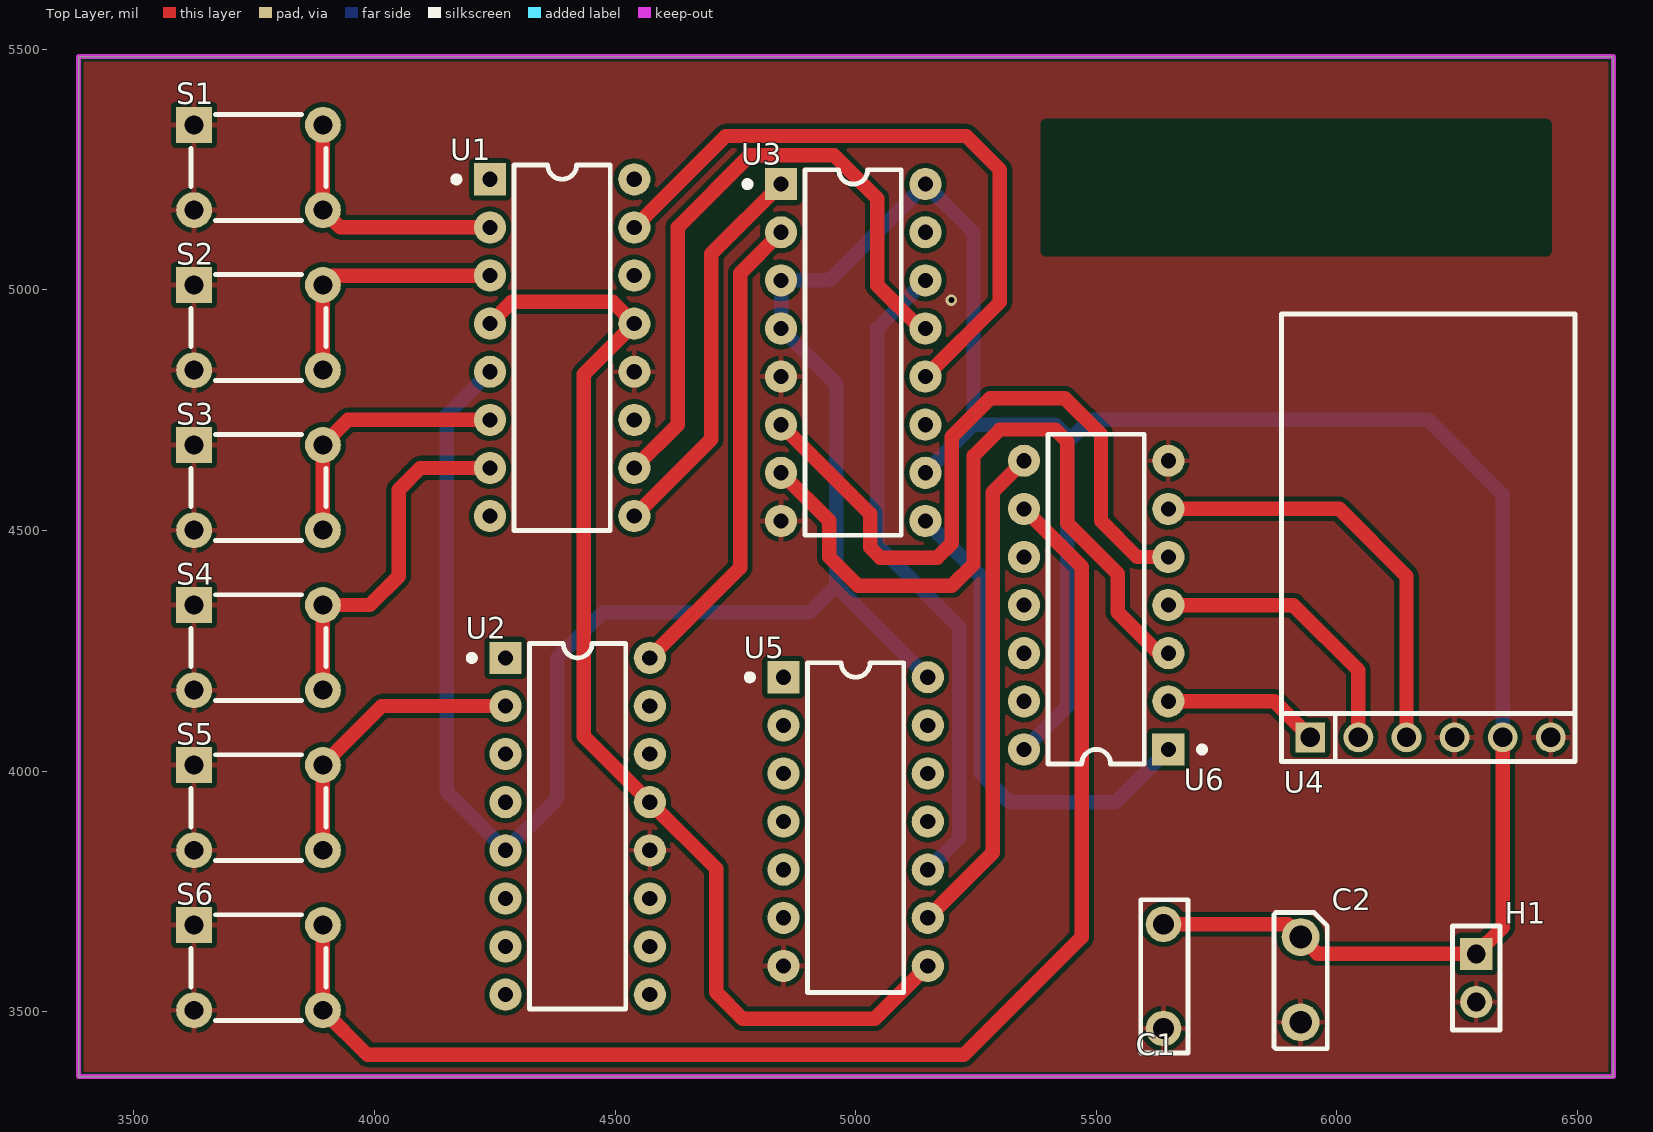
[diagram p0: Top Layer view]
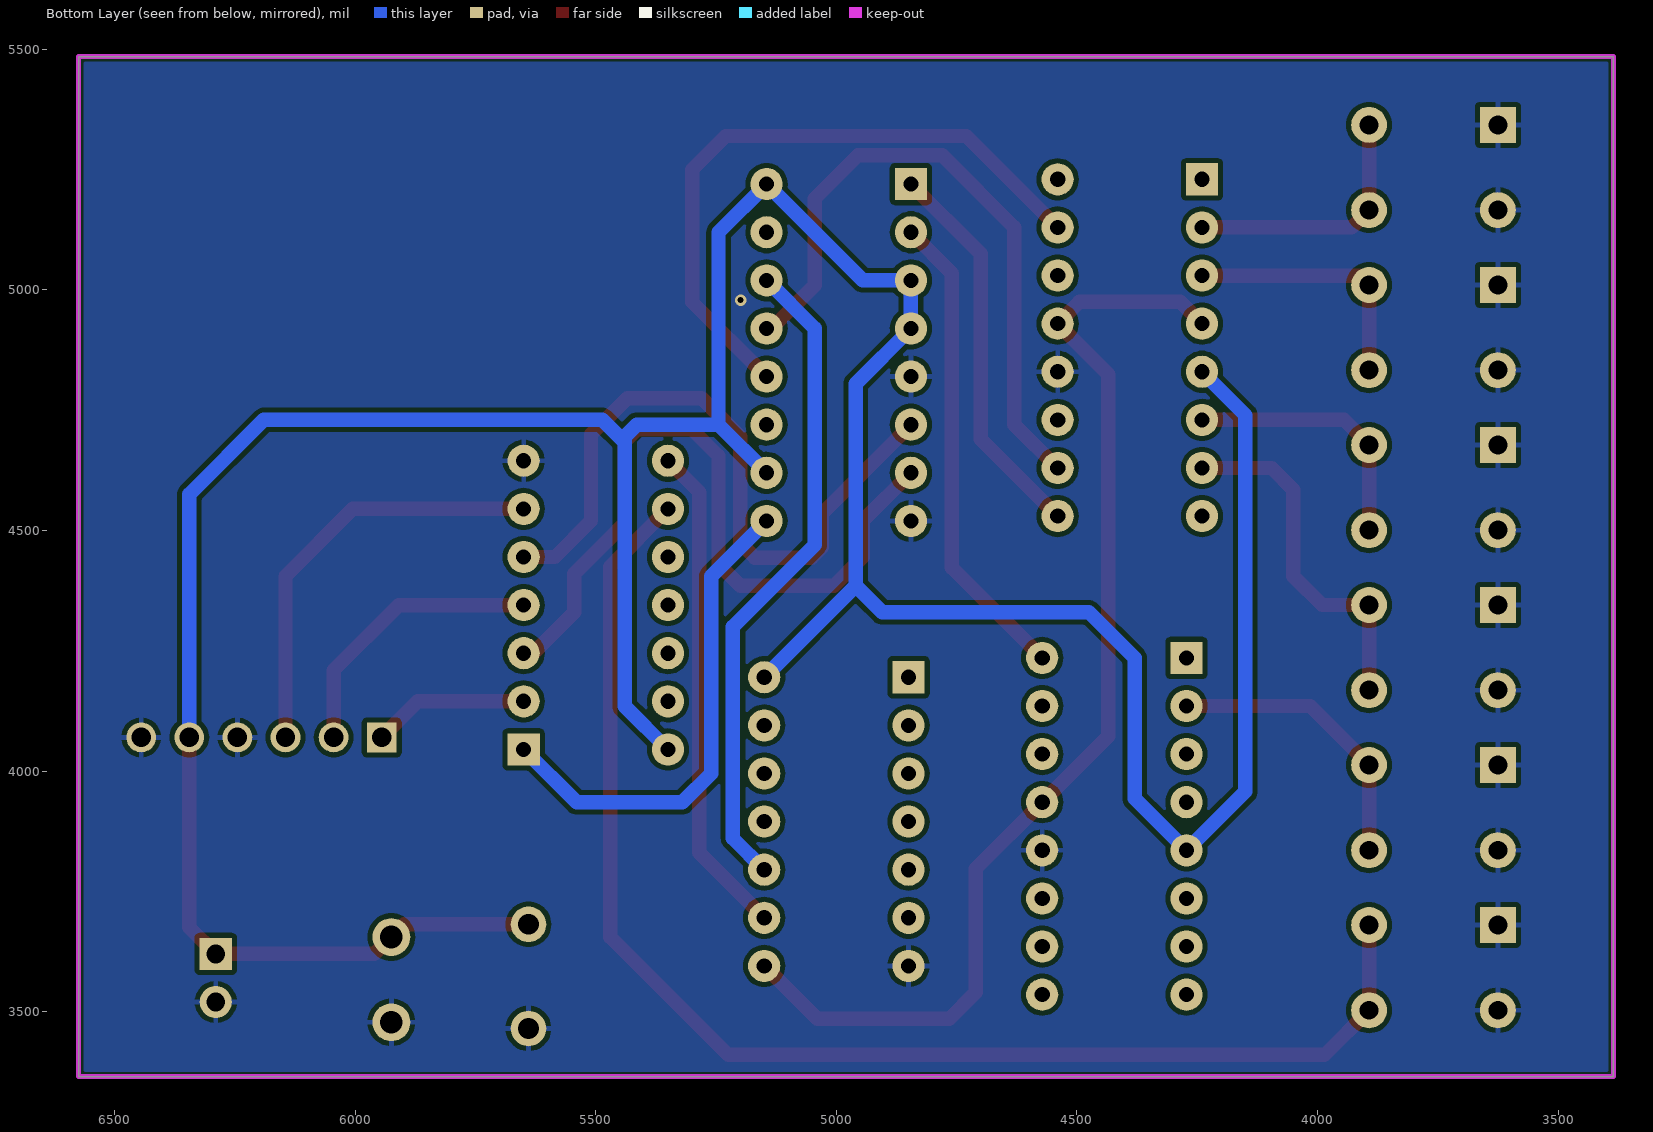
[diagram p1: Bottom Layer view, seen from below]
# Altium PCB MISC51507.pcbdoc
Units mil, origin at the board's own origin, x right, y up, seen from the top; angles counter-clockwise.
Board outline 3190 x 2120 mil, 2 copper layers (Top Layer, Bottom Layer), stack 62.206 mil thick; 15 components, 22 nets, 112 pads, 1 vias.

## Layer stack, top to bottom
Top Solder Mask Layer: solder mask 0.394, Dk 3.3
Top Layer: signal copper 1.379
Dielectric1: surface 59.449, FR4, Dk 4.5
Bottom Layer: signal copper 1.378
Bottom Solder Mask Layer: solder mask 0.394, Dk 3.3

## Board outline
3385,5485 3385,3365 6575,3365 6575,5485

## Design rules (kind name [scope] priority, off if disabled: settings)
BoardOutlineClearance copperThickness2oz_1 [All] p2 off: genericclearance=7.99 ignorepadtopadclearanceinfootprint=FALSE except(0: Arc-SplitContinuation Track-SplitContinuation SMDPad-SplitContinuation THPad-SplitContinuation Via-SplitContinuation Fill-SplitContinuation Region-SplitContinuation Poly-SplitContinuation Text-SplitContinuation Hole-SplitContinuation; 5.98: Arc-CutoutEdge SMDPad-CutoutEdge THPad-CutoutEdge Via-CutoutEdge Fill-CutoutEdge Region-CutoutEdge Text-CutoutEdge; 6.93: Hole-OutlineEdge Hole-CutoutEdge; 10: Poly-OutlineEdge Poly-CutoutEdge; 11.81: Arc-OutlineEdge Track-OutlineEdge SMDPad-OutlineEdge THPad-OutlineEdge Via-OutlineEdge Fill-OutlineEdge Region-OutlineEdge Text-OutlineEdge Track-CutoutEdge)
BoardOutlineClearance copperThickness1oz_1 [All] p4: genericclearance=4.02 ignorepadtopadclearanceinfootprint=FALSE except(0: Arc-SplitContinuation Track-SplitContinuation SMDPad-SplitContinuation THPad-SplitContinuation Via-SplitContinuation Fill-SplitContinuation Region-SplitContinuation Poly-SplitContinuation Text-SplitContinuation Hole-SplitContinuation; 6: SMDPad-CutoutEdge THPad-CutoutEdge Via-CutoutEdge Fill-CutoutEdge Region-CutoutEdge Text-CutoutEdge; 6.93: Hole-OutlineEdge Hole-CutoutEdge; 10: Poly-OutlineEdge Poly-CutoutEdge; 11.8: Arc-OutlineEdge Track-OutlineEdge SMDPad-OutlineEdge THPad-OutlineEdge Via-OutlineEdge Fill-OutlineEdge Region-OutlineEdge Text-OutlineEdge; 11.81: Arc-CutoutEdge Track-CutoutEdge)
Clearance copperThickness2oz [All] p1 off: gap=7.99 ignorepadtopadclearanceinfootprint=FALSE except(5.98: SMDPad-Track SMDPad-SMDPad THPad-Track SMDPad-THPad THPad-THPad Track-Via SMDPad-Via THPad-Via Via-Via Fill-Track Region-Track Fill-SMDPad Region-SMDPad Fill-THPad Region-THPad Fill-Via Region-Via Fill-Fill Fill-Region Region-Region Arc-Track Arc-SMDPad Arc-THPad Arc-Via Fill-Arc Region-Arc Arc-Arc Text-Track SMDPad-Text Text-THPad Text-Via Fill-Text Region-Text Arc-Text Text-Text; 6.93: Hole-Track Hole-SMDPad Hole-THPad Hole-Via Fill-Hole Region-Hole Hole-Arc Hole-Text; 10: Poly-Track Poly-SMDPad Poly-THPad Poly-Via Poly-Fill Poly-Region Poly-Poly Poly-Arc Poly-Text Poly-Hole)
Clearance copperThickness1oz [All] p3: gap=4.02 ignorepadtopadclearanceinfootprint=FALSE except(5.98: SMDPad-Track SMDPad-SMDPad THPad-Track SMDPad-THPad THPad-THPad Track-Via SMDPad-Via THPad-Via Via-Via Fill-Track Region-Track Fill-SMDPad Region-SMDPad Fill-THPad Region-THPad Fill-Via Region-Via Fill-Fill Fill-Region Region-Region; 6: Arc-Track Arc-SMDPad Arc-THPad Arc-Via Fill-Arc Region-Arc Arc-Arc Text-Track SMDPad-Text Text-THPad Text-Via Fill-Text Region-Text Arc-Text Text-Text; 6.93: Hole-Track Hole-SMDPad Hole-THPad Hole-Via Fill-Hole Region-Hole Hole-Arc Hole-Text; 10: Poly-Track Poly-SMDPad Poly-THPad Poly-Via Poly-Fill Poly-Region Poly-Poly Poly-Arc Poly-Text Poly-Hole)
Creepage creepage [All] p1: checkdistance=0 ignoreinternallayers=TRUE applytopolygonpour=TRUE
DiffPairsRouting differentialPair [All] p1: maxlimit=6 minlimit=6 mostfreqgap=6 toplayer_minwidth=5 toplayer_prefwidth=10 toplayer_maxwidth=100 toplayer_mingap=6 toplayer_prefgap=6 toplayer_maxgap=6 bottomlayer_minwidth=5 bottomlayer_prefwidth=10 bottomlayer_maxwidth=100 bottomlayer_mingap=6 bottomlayer_prefgap=6 bottomlayer_maxgap=6 maxuncoupledlength=10
HoleToHoleClearance otherClearance [All] p1: gap=11.81 allowstackedmicrovias=TRUE
Length netLength [All] p1: minlimit=0 maxlimit=0
MatchedLengths netLengthTolerance [All] p1: tolerance=1000
PasteMaskExpansion pasteMaskExpansion [All] p1: expansion=0
PlaneConnect innerPlane [All] p1: planeconnectstyle=Relief reliefexpansion=20 reliefentries=4 reliefconductorwidth=10 reliefairgap=10
PolygonConnect copperRegion [(InNet('GND'))] p1: connectstyle=Relief reliefconductorwidth=10 reliefentries=4 polygonreliefangle="90 Angle" airgapwidth=10 via.connectstyle=Relief via.reliefconductorwidth=10 via.reliefentries=4 via.polygonreliefangle="90 Angle" via.airgapwidth=10
RoutingVias viaSize [All] p1: holewidth=12.01 width=24.02 viastyle="Through Hole" minholewidth=11.81 minwidth=19.68 maxholewidth=248.03 maxwidth=393.7
SolderMaskExpansion solderMaskExpansion [IsVia] p1: expansion=-1000 istentingtop=TRUE
SolderMaskExpansion solderMaskExpansion [All] p2: expansion=2 istentingtop=FALSE
Width copperThickness2oz_2 [All] p1 off: maxlimit=100 minlimit=8 preferedwidth=10
Width copperThickness1oz_2 [All] p2: maxlimit=100 minlimit=5 preferedwidth=10

## Components (designator, comment, footprint, x,y, rotation, side; value= is the part's Value field where it differs from the comment)
C1 "0.1uF" CAP 5640,3465 r90 top
C2 "10uF" "CAP POL" 5925,3655 r270 top
H1 "" HDR-TH_2P-P2.54-V-F 6290,3570 r270 top
S1 "KEY" KEY-4 3625,5343.15 r0 top
S2 "KEY" KEY-4 3625,5010.52 r0 top
S3 "KEY" KEY-4 3625,4677.89 r0 top
S4 "KEY" KEY-4 3625,4345.26 r0 top
S5 "KEY" KEY-4 3625,4012.63 r0 top
S6 "KEY" KEY-4 3625,3680 r0 top
U1 "74LS75D" 74LS75D 4240,5230 r0 top
U2 "74LS75D" 74LS75D 4272.22,4235.29 r0 top
U3 "74LS148D" 74LS148D 4845,5220 r0 top
U4 "DCD_HEX" SMG 5945,4070 r0 top
U5 "74LS32" 74LS32 4850,4195 r0 top
U6 "74LS04" 74LS04 5650,4045 r180 top

## Footprints (in the part's own frame and the unit in brackets; to place one, negate y for a bottom-side part, rotate by r counter-clockwise, add the part's x,y. Pads: shape width x height; smd on the part's side, far side on the other; paste and mask are expansions set on the pad)
74LS04 [mm]
  rect 1.7x1.7 hole 0.8 paste+0 mask+0.102: 1(0,0)
  round 1.7 hole 0.8 paste+0 mask+0.102: 2(0,-2.54) 3(0,-5.08) 4(0,-7.62) 5(0,-10.16) 6(0,-12.7) 7(0,-15.24) 8(7.62,-15.24) 9(7.62,-12.7) 10(7.62,-10.16) 11(7.62,-7.62) 12(7.62,-5.08) 13(7.62,-2.54) 14(7.62,0)
  silkscreen extent -1.9,-16.64 6.35,0.76
74LS32 [mm]
  rect 1.7x1.7 hole 0.8 paste+0 mask+0.102: 1(0,0)
  round 1.7 hole 0.8 paste+0 mask+0.102: 2(0,-2.54) 3(0,-5.08) 4(0,-7.62) 5(0,-10.16) 6(0,-12.7) 7(0,-15.24) 8(7.62,-15.24) 9(7.62,-12.7) 10(7.62,-10.16) 11(7.62,-7.62) 12(7.62,-5.08) 13(7.62,-2.54) 14(7.62,0)
  silkscreen extent -1.9,-16.64 6.35,0.76
74LS75D [mm]
  rect 1.7x1.7 hole 0.8 paste+0 mask+0.102: 1(0,0)
  round 1.7 hole 0.8 paste+0 mask+0.102: 2(0,-2.54) 3(0,-5.08) 4(0,-7.62) 5(0,-10.16) 6(0,-12.7) 7(0,-15.24) 8(0,-17.78) 9(7.62,-17.78) 10(7.62,-15.24) 11(7.62,-12.7) 12(7.62,-10.16) 13(7.62,-7.62) 14(7.62,-5.08) 15(7.62,-2.54) 16(7.62,0)
  silkscreen extent -1.9,-18.54 6.35,0.76
74LS148D [mm]
  rect 1.7x1.7 hole 0.8 paste+0 mask+0.102: 1(0,0)
  round 1.7 hole 0.8 paste+0 mask+0.102: 2(0,-2.54) 3(0,-5.08) 4(0,-7.62) 5(0,-10.16) 6(0,-12.7) 7(0,-15.24) 8(0,-17.78) 9(7.62,-17.78) 10(7.62,-15.24) 11(7.62,-12.7) 12(7.62,-10.16) 13(7.62,-7.62) 14(7.62,-5.08) 15(7.62,-2.54) 16(7.62,0)
  silkscreen extent -1.9,-18.54 6.35,0.76
CAP [mm]
  round 1.88 hole 1.1 paste+0 mask+0.102: 1(0,0) 2(5.5,0)
  silkscreen extent -1.3,-1.3 6.8,1.2
"CAP POL" [mm]
  round 2 hole 1.2 paste+0 mask+0.102: 1(0,0) 2(4.5,0)
  silkscreen extent -1.3,-1.4 5.9,1.4
HDR-TH_2P-P2.54-V-F [mm]
  rect 1.7x1.7 hole 1: 1(-1.27,0)
  round 1.7 hole 1: 2(1.27,0)
  silkscreen extent -2.74,-1.25 2.74,1.25
KEY-4 [mm]
  rect 1.9x1.9 hole 1 paste+0 mask+0.102: 1(0,0)
  round 1.9 hole 1 paste+0 mask+0.102: 2(6.8,0) 3(0,-4.5) 4(6.8,-4.5)
  silkscreen extent -0.16,-5.04 6.96,0.54
SMG [mil]
  rect 62x62 hole 40.16 paste+0 mask+4: 1(0,0)
  round 62 hole 40.16 paste+0 mask+4: 2(100,0) 3(200,0) 4(300,0) 5(400,0) 6(500,0)
  silkscreen extent -60,-50 550,50

## Via types
v1: diameter 24.02, hole 12, Top Layer to Bottom Layer, 1 vias

## Nets (pads, with @x,y where several pads share a name; then routed paths per layer and width w, separated by ;. In a path a pad name is that pad's centre, name@x,y a point inside that pad or via, vN(x,y) a via of type N, cw(c..) or ccw(c..) an arc to the next point about the centre after c; other vN are vias at no path point)
$2N7: S1.2 S1.4 U1.2 | length 539.4
  Top Layer w30: S1.2 S1.4 3928.7,5130 U1.2
$2N8: S2.2 S2.4 U1.3 | length 532.5
  Top Layer w30: S2.4 S2.2 3912.2,5030 U1.3
$2N9: S3.2 S3.4 U1.6 | length 546
  Top Layer w30: S3.4 S3.2 3944.83,4730 U1.6
$2N10: S4.2 S4.4 U1.7 | length 747.8
  Top Layer w30: S4.4 S4.2 3990.26,4345.26 4050,4405 4050,4585 4095,4630 U1.7
$2N11: S5.2 S5.4 U2.2 | length 607.5
  Top Layer w30: S5.4 S5.2 4015.38,4135.29 U2.2
$2N12: U1.16
$2N13: U1.15 U3.12 | length 1361.9
  Top Layer w30: U1.15 4730,5320 5230,5320 5300,5250 5300,4975 U3.12
$2N14: U1.10 U3.13 | length 1369
  Top Layer w30: U1.10 4630,4720 4630,5130 4780,5280 4955,5280 5045,5190 5045,5010 5135,4920 U3.13
$2N15: U1.9 U3.1 | length 816.3
  Top Layer w30: U1.9 4700,4690 4700,5075 U3.1
$2N16: U2.16 U3.2 | length 997.7
  Top Layer w30: U2.16 4760,4423.07 4760,5035 U3.2
$2N17: U3.9 U6.1 | length 1033.1
  Bottom Layer w30: U3.9 5260,4405 5260,3995 5320,3935 5540,3935 U6.1
$2N18: U3.7 U6.3 | length 1551.8
  Top Layer w30: U3.7 4945,4520 4945,4445 5005,4385 5200,4385 5245,4430 5245,4655 5300,4710 5415,4710 5440,4685 5440,4515 5545,4410 5545,4330 5630,4245 U6.3
$2N19: U3.6 U6.5 | length 1469.3
  Top Layer w30: U3.6 5030,4535 5030,4465 5051.21,4443.79 5170,4443.79 5200,4473.79 5200,4695 5280,4775 5435,4775 5510,4700 5510,4520 5585,4445 U6.5
$2N20: U3.14 U5.10 | length 1363.8
  Bottom Layer w30: U3.14 5045,4920 5045,4470 5215,4300 5215,3860 U5.10
$2N21: U1.4 U1.13 U2.13 U5.8 | length 2393.2
  Top Layer w30: U1.4 4285.25,4975.25 4494.75,4975.25 U1.13 4435,4825 4435,4072.51 U2.13 4710,3797.51 4710,3540 4765,3485 5040,3485 U5.8
$2N32: U4.1 U6.2 | length 326.1
  Top Layer w30: U6.2 5870,4145 U4.1
$2N33: U4.2 U6.4 | length 590.9
  Top Layer w30: U6.4 5910,4345 6045,4210 U4.2
$2N34: U4.3 U6.6 | length 888
  Top Layer w30: U6.6 6005,4545 6145,4405 U4.3
$2N35: S6.2 S6.4 U6.9 | length 2834.1
  Top Layer w30: S6.2 S6.4 3985.55,3410 5225,3410 5470,3655 5470,4425 U6.9
$2N36: U5.9 U6.8 | length 1032.8
  Top Layer w30: U5.9 5285,3830 5285,4580 U6.8
GND: C1.1 C2.2 H1.2 S1.1 S1.3 S2.1 S2.3 S3.1 S3.3 S4.1 S4.3 S5.1 S5.3 S6.1 S6.3 U1.12 U2.12 U3.5 U3.8 U4.4 U4.6 U5.7 U6.7
  other v1: 5199.1,4979.1
VCC: C1.2 C2.1 H1.1 U1.5 U2.5 U3.3 U3.4 U3.10 U3.16 U4.5 U5.14 U6.14 | length 7720.6
  Top Layer w30: C1.2 5898.46,3681.54 C2.1 5960,3620 H1.1 6345,3675 U4.5
  Bottom Layer w30: U1.5 4150,4740 4150,3957.51 U2.5 4380,3943.07 4380,4235 4475,4330 4905,4330 4960,4385 ; U3.10 5245,4720 ; U5.14 4960,4385 ; U6.14 5440,4135 5440,4683.29 ; U4.5 6345,4575 6190,4730 5486.71,4730 5440,4683.29 ; 4960,4385 4960,4805 U3.4 U3.3 4945,5020 U3.16 5245,5120 5245,4720 ; 5245,4720 5415,4720 5440,4695 5440,4683.29
pads on no net: U1.1 U1.8 U1.11 U1.14 U2.1 U2.3 U2.4 U2.6 U2.7 U2.8 U2.9 U2.10 U2.11 U2.14 U2.15 U3.11 U3.15 U5.1 U5.2 U5.3 U5.4 U5.5 U5.6 U5.11 U5.12 U5.13 U6.10 U6.11 U6.12 U6.13

## Polygon pours and split planes (outlines as drawn)
GND on Top Layer (solid, remove dead copper, pour order 0): 3000,5690 3000,3000 6900,3000 6900,5690
GND on Bottom Layer (solid, remove dead copper, pour order 2): 3145,5655 3145,3170 6910,3170 6910,5655

## Keep-outs
Board Outline Layer:
  the board outline again, w10

## Silkscreen, mask and mechanical layers (free items; w line width, h text height)
Top Silkscreen Layer:
  lines w10: 5885.16,4020 5885.16,4950 6495,4950 6495,4020 5885.16,4020